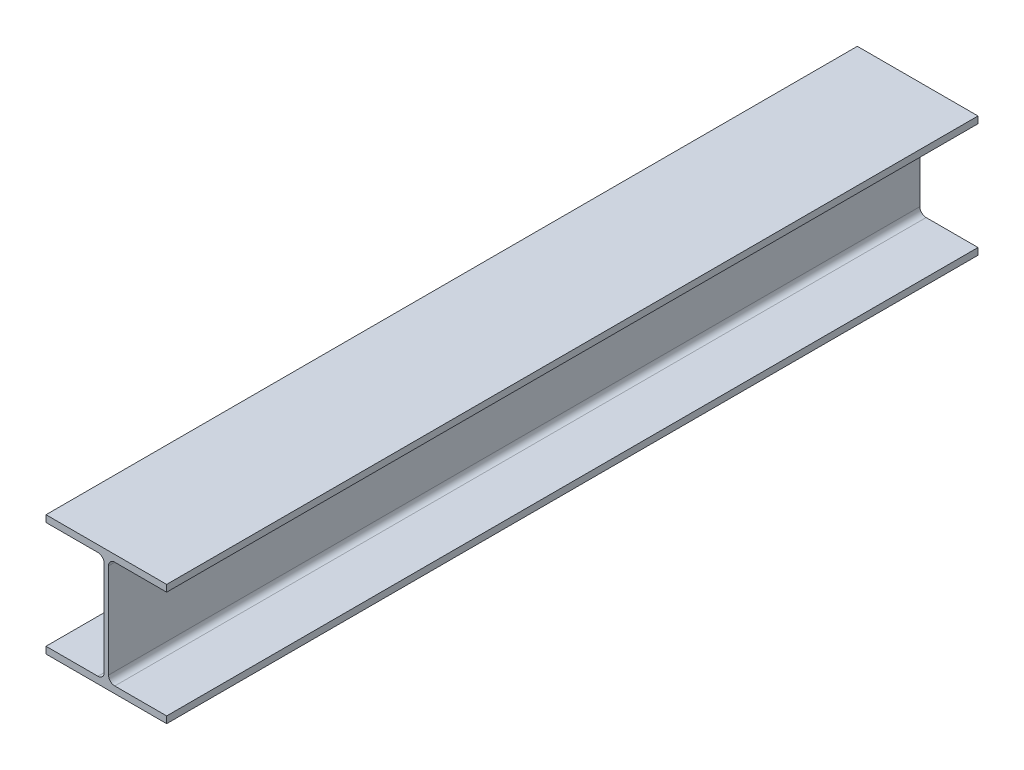
SolidWorks part; units mm, degrees
material "Q235"
ref_plane "Front Plane" through (0, 0, 0) normal (0, 0, 1) x (1, 0, 0)
ref_plane "Top Plane" through (0, 0, 0) normal (0, 1, 0) x (1, 0, 0)
ref_plane "Right Plane" through (0, 0, 0) normal (1, 0, 0) x (0, 0, -1)
sketch "Sketch1" plane through (0, 0, 0) normal (0, 0, 1) x (1, 0, 0)
  line L0 (0, 0) -> (250, 0)
  line L1 (250, 0) -> (250, 14)
  line L2 (250, 14) -> (142.5, 14)
  line L3 (129.5, 27) -> (129.5, 223)
  line L4 (142.5, 236) -> (250, 236)
  line L5 (250, 236) -> (250, 250)
  line L6 (250, 250) -> (0, 250)
  line L7 (0, 250) -> (0, 236)
  line L8 (0, 236) -> (107.5, 236)
  line L9 (120.5, 223) -> (120.5, 27)
  line L10 (107.5, 14) -> (0, 14)
  line L11 (0, 14) -> (0, 0)
  line L12 (125, 250) -> (125, 0) construction
  arc A0 (142.5, 14) -> (129.5, 27) centre (142.5, 27) cw
  arc A1 (120.5, 27) -> (107.5, 14) centre (107.5, 27) cw
  arc A2 (129.5, 223) -> (142.5, 236) centre (142.5, 223) cw
  arc A3 (107.5, 236) -> (120.5, 223) centre (107.5, 223) cw
  point P21 (129.5, 236)
  dimension "D7" = 13
  dimension "D1" = 250
  dimension "D2" = 250
  dimension "D3" = 9
  dimension "D4" = 4.5
  dimension "D5" = 14
  dimension "D6" = 14
extrude "Boss-Extrude1" add sketch "Sketch1" along normal blind 1681
sketch "Sketch2" plane through (0, 250, 0) normal (0, 1, 0) x (1, 0, 0)
  line L0 (125, -1681) -> (125, 0) construction
  line L1 (250, -1681) -> (0, -1681) construction
  line L2 (250, 0) -> (0, 0) construction
